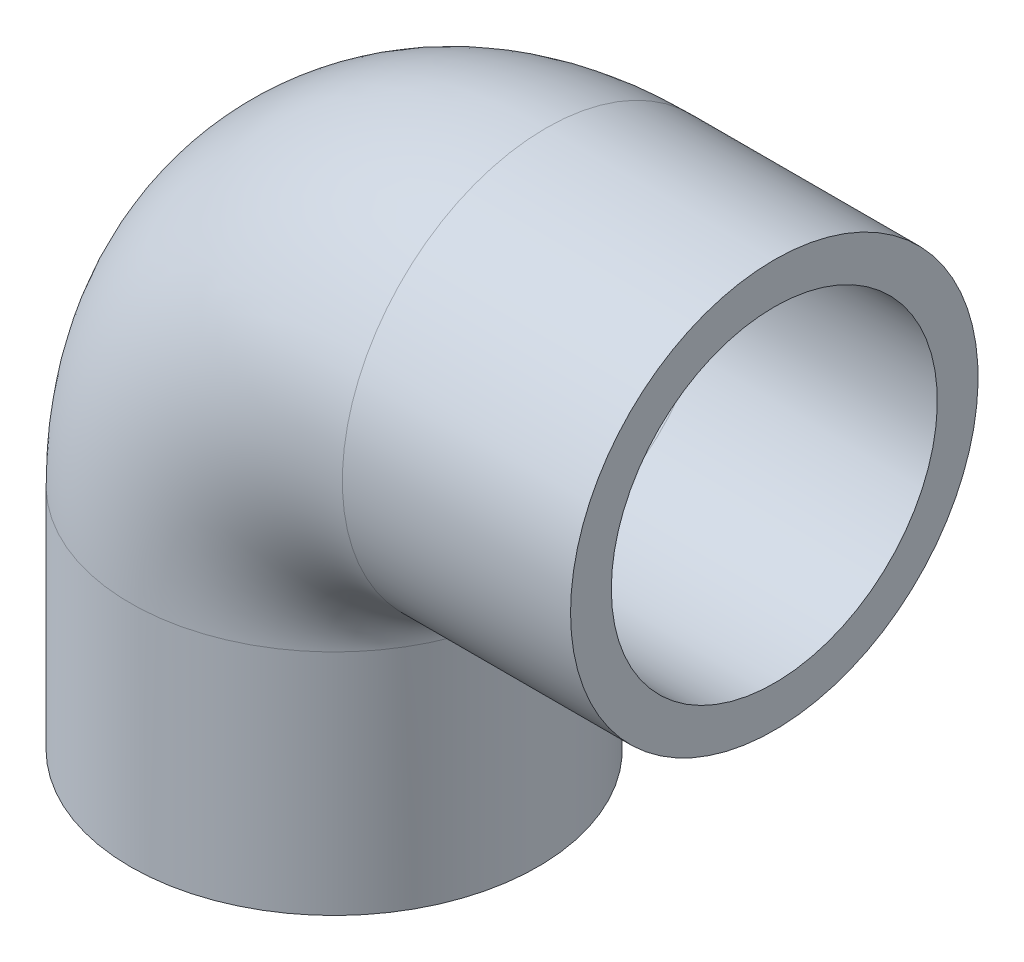
from build123d import *

# Parameters (mm, degrees)
SKETCH_2_R   = 12.5
SKETCH_2_R_2 = 10


with BuildPart() as part:
    # 扫描1: sweep along a path in 草图1
    with BuildLine(Plane.XY) as sweep_1_path:
        Line((0, 0), (0, 14))
        ThreePointArc((0, 14), (3.807611845, 23.192388155), (13, 27))
        Line((13, 27), (27, 27))
    # 草图2 → 扫描1 (sweep)
    with BuildSketch(Plane(origin=(0, 0, 0), x_dir=(1, 0, 0), z_dir=(0, 1, 0))):
        Circle(SKETCH_2_R)
        Circle(SKETCH_2_R_2, mode=Mode.SUBTRACT)
    sweep(path=sweep_1_path.line)


solid = part.part
